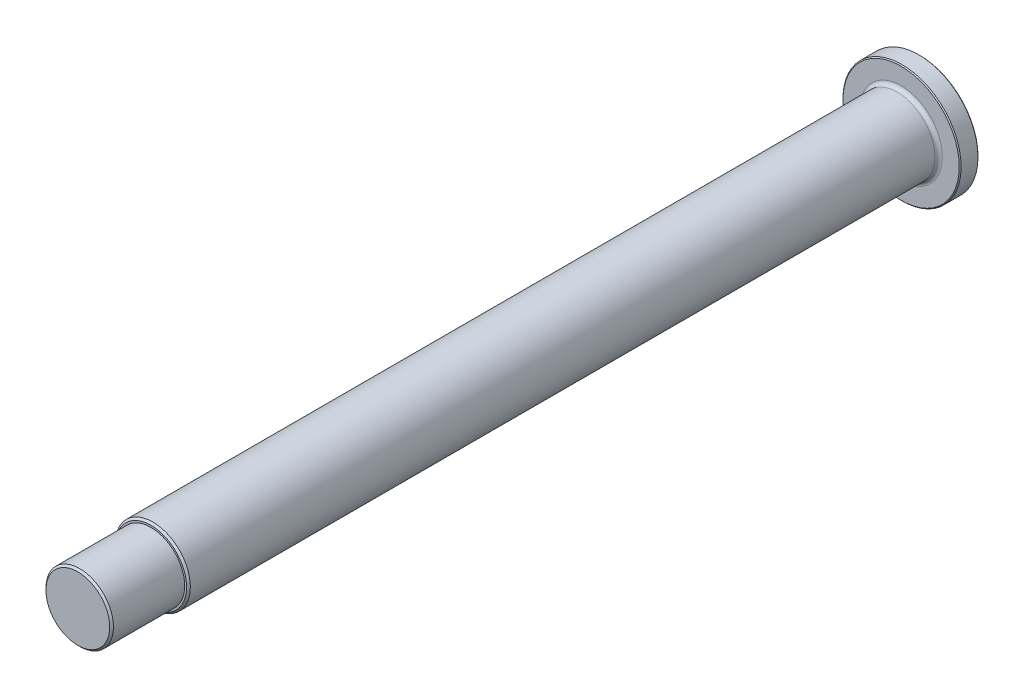
from build123d import *

# Parameters (mm, degrees)
SKETCH_1_R      = 31.5
EXTRUDE_1_DEPTH = 10
SKETCH_2_R      = 20
EXTRUDE_2_DEPTH = 400
SKETCH_3_R      = 18
EXTRUDE_3_DEPTH = 39
FILLET_1_R      = 2
CHAMFER_2_SIZE  = 1
CHAMFER_3_SIZE  = 0.5


with BuildPart() as part:
    # 草图1 → 凸台-拉伸1 (new body)
    with BuildSketch(Plane.XY):
        Circle(SKETCH_1_R)
    extrude(amount=EXTRUDE_1_DEPTH)

    # 草图2 → 凸台-拉伸2 (add)
    with BuildSketch(Plane.XY.offset(10)):
        Circle(SKETCH_2_R)
    extrude(amount=EXTRUDE_2_DEPTH)

    # 草图3 → 凸台-拉伸3 (add)
    with BuildSketch(Plane.XY.offset(410)):
        Circle(SKETCH_3_R)
    extrude(amount=EXTRUDE_3_DEPTH)

    # 圆角1
    fillet_1_edges = [part.edges().sort_by_distance(p)[0] for p in [
        (-20, 0, 10),
    ]]
    fillet(fillet_1_edges, radius=FILLET_1_R)

    # 倒角2
    chamfer_2_edges = [part.edges().sort_by_distance(p)[0] for p in [
        (-18, 0, 449),
        (-20, 0, 410),
    ]]
    chamfer(chamfer_2_edges, length=CHAMFER_2_SIZE)

    # 倒角3
    chamfer_3_edges = [part.edges().sort_by_distance(p)[0] for p in [
        (-31.5, 0, 0),
        (-31.5, 0, 10),
    ]]
    chamfer(chamfer_3_edges, length=CHAMFER_3_SIZE)


solid = part.part
